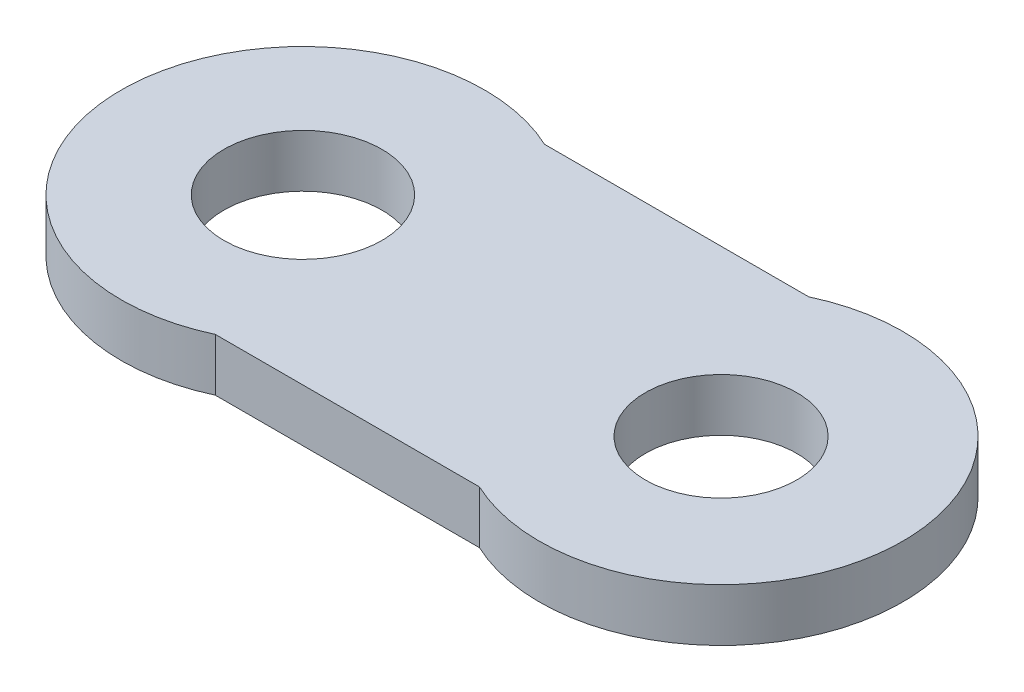
SolidWorks part; units mm, degrees
ref_plane "前视基准面" through (0, 0, 0) normal (0, 0, 1) x (1, 0, 0)
ref_plane "上视基准面" through (0, 0, 0) normal (0, 1, 0) x (1, 0, 0)
ref_plane "右视基准面" through (0, 0, 0) normal (1, 0, 0) x (0, 0, -1)
sketch "草图1" plane through (0, 0, 0) normal (0, 1, 0) x (1, 0, 0)
  line L3 (-1.0799, 2.5) -> (2.9312, 2.5)
  line L4 (-1.0799, -2.5) -> (2.9312, -2.5)
  arc A0 (-1.0799, 2.5) -> (-1.0799, -2.5) centre (-2.2493, 0) ccw
  circle A1 centre (-2.2493, 0) radius 1.2
  arc A2 (2.9312, -2.5) -> (2.9312, 2.5) centre (4.1007, 0) ccw
  circle A3 centre (4.1007, 0) radius 1.15
  dimension "D1" = 5.52
  dimension "D2" = 2.4
  dimension "D6" = 5.52
  dimension "D7" = 2.3
  dimension "D3" = 6.35
extrude "凸台-拉伸1" add sketch "草图1" along normal blind 0.8
